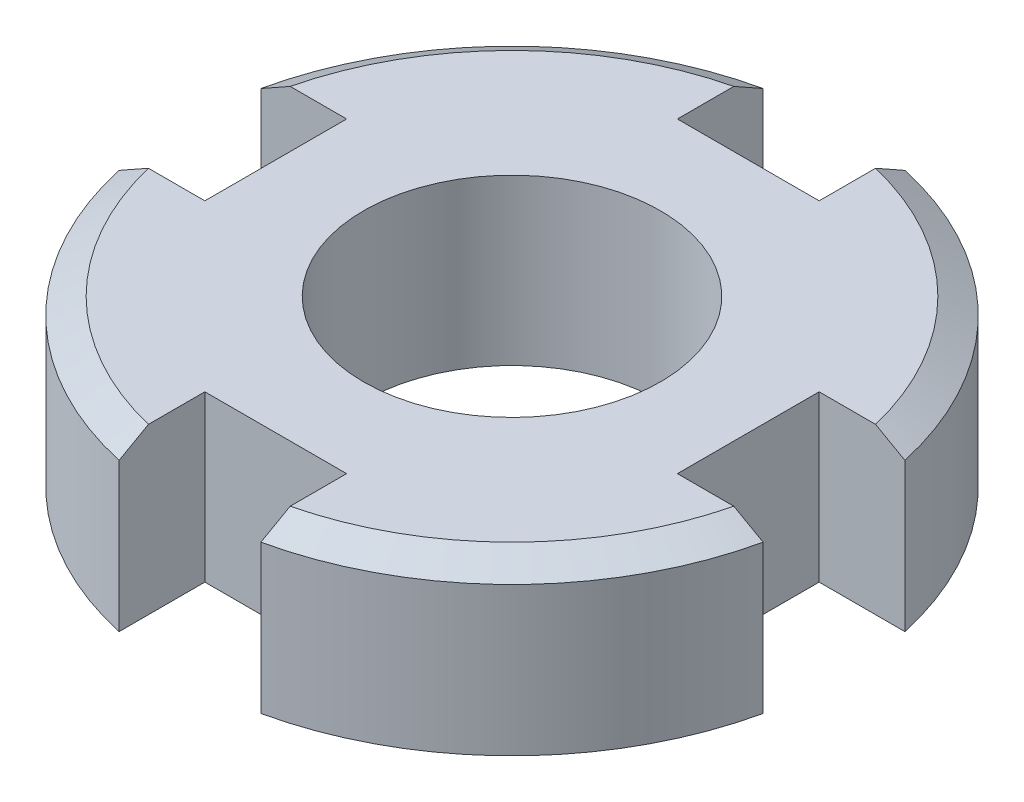
from build123d import *
from OCP.BRepFilletAPI import BRepFilletAPI_MakeChamfer

# Parameters (mm, degrees)
EXTRUDE_1_DEPTH = 5
M10X1_0_1_D     = 9
CHAMFER_1_SIZE  = 0.5
CHAMFER_1_SIZE2 = 0.866025404


with BuildPart() as part:
    # 草图1 → 凸台-拉伸1 (new body)
    with BuildSketch(Plane(origin=(0, 0, 0), x_dir=(1, 0, 0), z_dir=(0, 1, 0))):
        with BuildLine():
            Line((-2.15, 9.766140486), (-2.15, 7.166140486))
            Line((-2.15, 7.166140486), (2.15, 7.166140486))
            Line((2.15, 7.166140486), (2.15, 9.766140486))
            ThreePointArc((2.15, 9.766140486), (7.071067812, 7.071067812), (9.766140486, 2.15))
            Line((9.766140486, 2.15), (7.166140486, 2.15))
            Line((7.166140486, 2.15), (7.166140486, -2.15))
            Line((7.166140486, -2.15), (9.766140486, -2.15))
            ThreePointArc((9.766140486, -2.15), (7.071067812, -7.071067812), (2.15, -9.766140486))
            Line((2.15, -9.766140486), (2.15, -7.166140486))
            Line((2.15, -7.166140486), (-2.15, -7.166140486))
            Line((-2.15, -7.166140486), (-2.15, -9.766140486))
            ThreePointArc((-2.15, -9.766140486), (-7.071067812, -7.071067812), (-9.766140486, -2.15))
            Line((-9.766140486, -2.15), (-7.166140486, -2.15))
            Line((-7.166140486, -2.15), (-7.166140486, 2.15))
            Line((-7.166140486, 2.15), (-9.766140486, 2.15))
            ThreePointArc((-9.766140486, 2.15), (-7.071067812, 7.071067812), (-2.15, 9.766140486))
        make_face()
    extrude(amount=EXTRUDE_1_DEPTH)

    # M10x1.0 螺纹孔1 (through all)
    with Locations(Plane(origin=(0, 5, 0), x_dir=(1, 0, 0), z_dir=(0, 1, 0))):
        with Locations((0, 0)):
            Hole(M10X1_0_1_D / 2)

    # 倒角1: one chamfer whose edges measure the first distance from different faces: ONE call of the kernel's chamfer builder (chamfer() names one face for all edges)
    chamfer_1_edges_1 = [part.edges().sort_by_distance(p)[0] for p in [
        (-7.071067812, 5, 7.071067812),
    ]]
    chamfer_1_side_1 = [part.faces().sort_by_distance(p)[0] for p in [
        (-7.071067812, 2.5, 7.071067812),
    ]]
    chamfer_1_edges_2 = [part.edges().sort_by_distance(p)[0] for p in [
        (7.071067812, 5, 7.071067812),
    ]]
    chamfer_1_side_2 = [part.faces().sort_by_distance(p)[0] for p in [
        (7.071067812, 2.5, 7.071067812),
    ]]
    chamfer_1_edges_3 = [part.edges().sort_by_distance(p)[0] for p in [
        (-7.071067812, 5, -7.071067812),
    ]]
    chamfer_1_side_3 = [part.faces().sort_by_distance(p)[0] for p in [
        (-7.071067812, 2.5, -7.071067812),
    ]]
    chamfer_1_edges_4 = [part.edges().sort_by_distance(p)[0] for p in [
        (7.071067812, 5, -7.071067812),
    ]]
    chamfer_1_side_4 = [part.faces().sort_by_distance(p)[0] for p in [
        (7.071067812, 2.5, -7.071067812),
    ]]
    chamfer_1 = BRepFilletAPI_MakeChamfer(part.part.solid().wrapped)
    for e in chamfer_1_edges_1:
        chamfer_1.Add(CHAMFER_1_SIZE, CHAMFER_1_SIZE2, e.wrapped, chamfer_1_side_1[0].wrapped)  # the first distance lies on this face
    for e in chamfer_1_edges_2:
        chamfer_1.Add(CHAMFER_1_SIZE, CHAMFER_1_SIZE2, e.wrapped, chamfer_1_side_2[0].wrapped)  # the first distance lies on this face
    for e in chamfer_1_edges_3:
        chamfer_1.Add(CHAMFER_1_SIZE, CHAMFER_1_SIZE2, e.wrapped, chamfer_1_side_3[0].wrapped)  # the first distance lies on this face
    for e in chamfer_1_edges_4:
        chamfer_1.Add(CHAMFER_1_SIZE, CHAMFER_1_SIZE2, e.wrapped, chamfer_1_side_4[0].wrapped)  # the first distance lies on this face
    add(Compound.cast(chamfer_1.Shape()), mode=Mode.REPLACE)


solid = part.part
